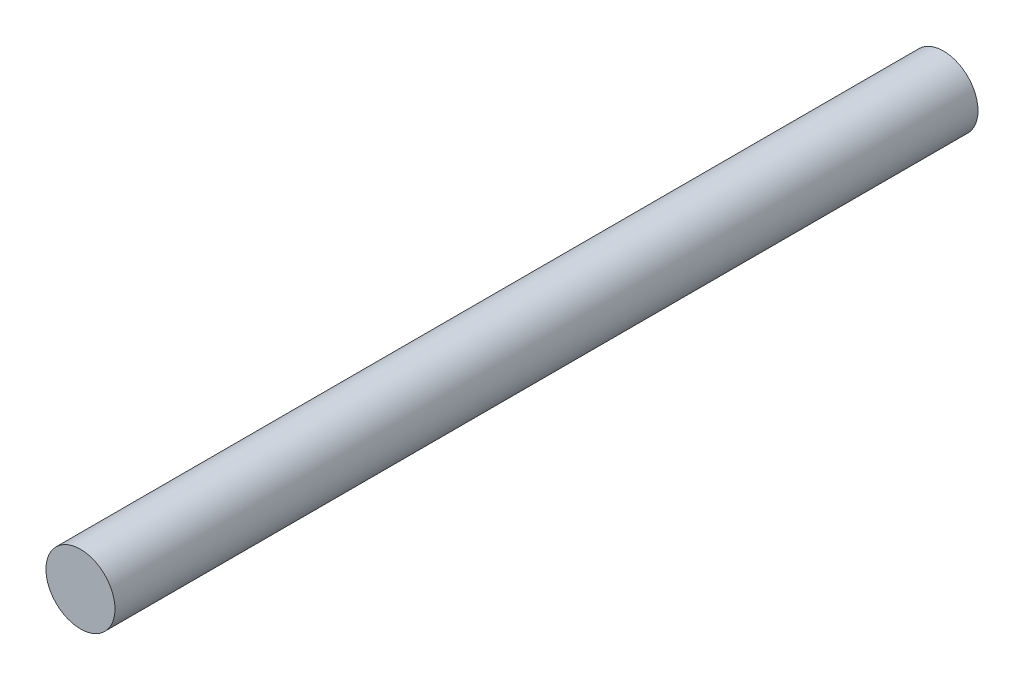
SolidWorks part; units mm, degrees
ref_plane "前视基准面" through (0, 0, 0) normal (0, 0, 1) x (1, 0, 0)
ref_plane "上视基准面" through (0, 0, 0) normal (0, 1, 0) x (1, 0, 0)
ref_plane "右视基准面" through (0, 0, 0) normal (1, 0, 0) x (0, 0, -1)
sketch "草图1" plane through (0, 0, 0) normal (0, 0, 1) x (1, 0, 0)
  circle A0 centre (0, 0) radius 6
  dimension "D1" = 12
extrude "凸台-拉伸1" add sketch "草图1" along normal mid plane 150
